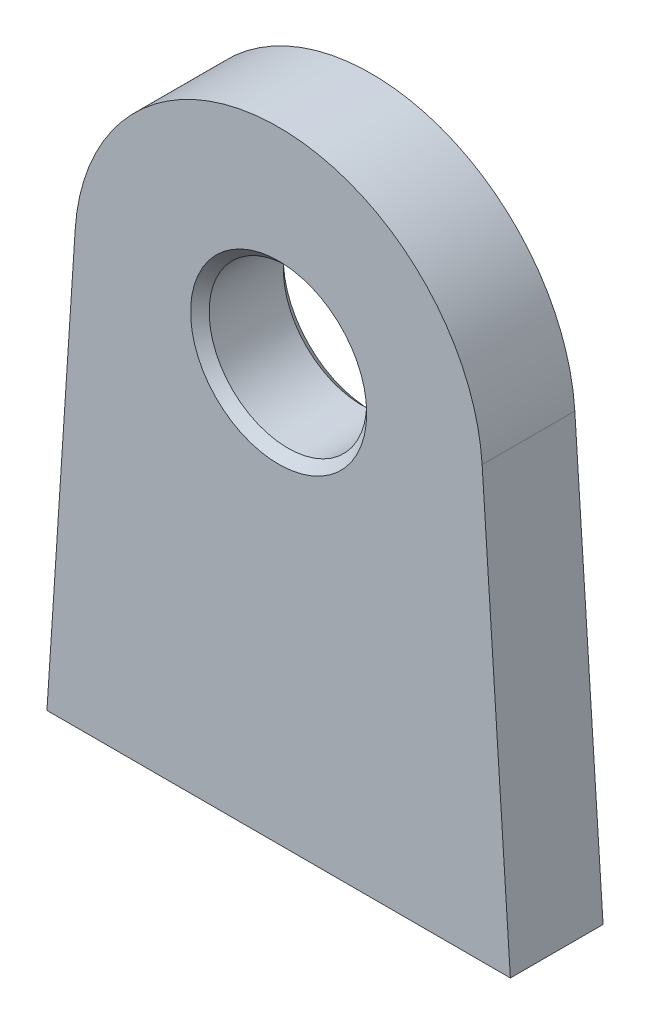
from build123d import *

# Parameters (mm, degrees)
SKETCH1_R           = 8.5
BOSS_EXTRUDE1_DEPTH = 10
CHAMFER1_SIZE       = 1


with BuildPart() as part:
    # Sketch1 → Boss-Extrude1 (new body)
    with BuildSketch(Plane.XY):
        with BuildLine():
            Line((0, 0), (50, 0))
            Line((50, 0), (46.952793231, 46.440440684))
            ThreePointArc((46.952793231, 46.440440684), (25, 67), (3.047206769, 46.440440684))
            Line((3.047206769, 46.440440684), (0, 0))
        make_face()
        with Locations((25, 45)):
            Circle(SKETCH1_R, mode=Mode.SUBTRACT)
    extrude(amount=BOSS_EXTRUDE1_DEPTH)

    # Chamfer1
    chamfer1_edges = [part.edges().sort_by_distance(p)[0] for p in [
        (16.5, 45, 0),
        (16.5, 45, 10),
    ]]
    chamfer(chamfer1_edges, length=CHAMFER1_SIZE)


solid = part.part
